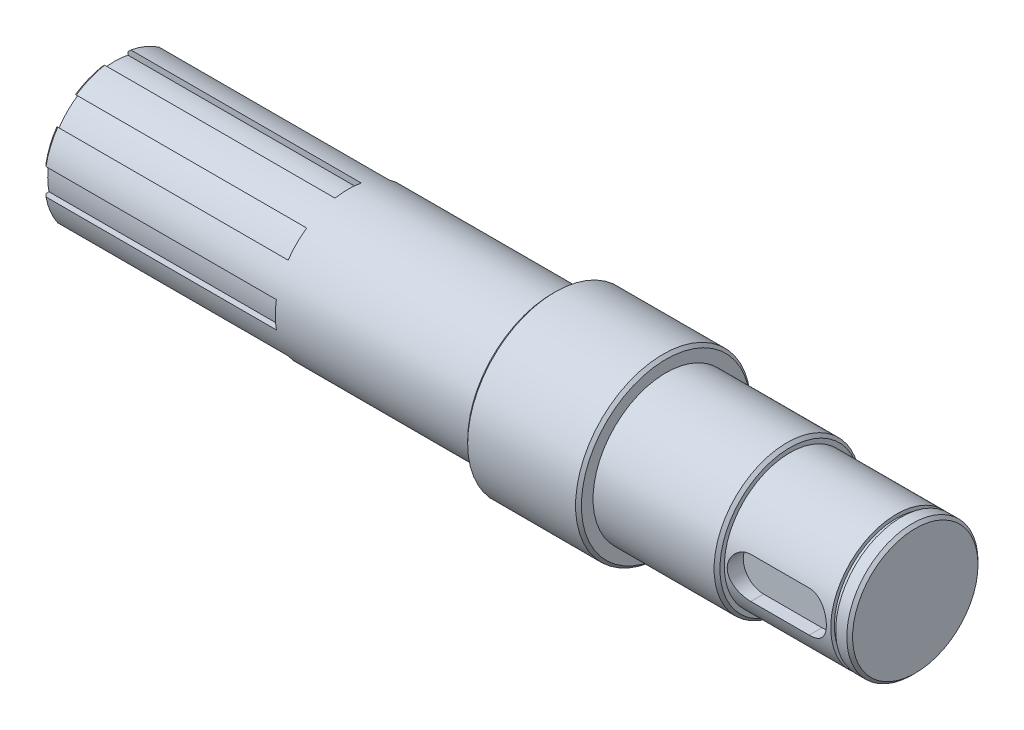
from build123d import *

# Parameters (mm, degrees)
CHAMFER_1_SIZE      = 1
CUT_EXTRUDE_START   = 1.7
SKETCH_2_R          = 22.5
SKETCH_2_R_2        = 21.25
CUT_EXTRUDE_1_DEPTH = 1.7
CUT_EXTRUDE_2_DEPTH = 5.5
CUT_EXTRUDE_START_2 = -80
CUT_EXTRUDE_3_DEPTH = 80
CHAMFER_2_SIZE      = 1


with BuildPart() as part:
    # 草图1 → 旋转1 (revolve)
    with BuildSketch(Plane.XY, mode=Mode.PRIVATE) as revolve_1_sk:
        Polygon((0, 0), (0, 25), (150, 25), (150, 30), (189, 30), (189, 25), (231.5, 25), (231.5, 22.5), (274.5, 22.5), (274.5, 0), align=None)
    revolve(revolve_1_sk.sketch.rotate(Axis((274.5, 0, 0), (-1, 0, 0)), 90), axis=Axis((274.5, 0, 0), (-1, 0, 0)))

    # 倒角1
    chamfer_1_edges = [part.edges().sort_by_distance(p)[0] for p in [
        (274.5, 0, 22.5),
        (231.5, 0, 25),
        (189, 0, 30),
        (150, 0, 30),
    ]]
    chamfer(chamfer_1_edges, length=CHAMFER_1_SIZE)

    # 草图2 → 切除-拉伸1 (cut)
    with BuildSketch(Plane(origin=(268, 0, 0), x_dir=(0, 0, -1), z_dir=(1, 0, 0)).offset(CUT_EXTRUDE_START)):
        Circle(SKETCH_2_R)
        Circle(SKETCH_2_R_2, mode=Mode.SUBTRACT)
    extrude(amount=-CUT_EXTRUDE_1_DEPTH, mode=Mode.SUBTRACT)

    # 草图3 → 切除-拉伸2 (cut)
    with BuildSketch(Plane.XY.offset(22.5)):
        with BuildLine():
            Line((239.5, 7), (259.5, 7))
            ThreePointArc((259.5, 7), (266.5, 0), (259.5, -7))
            Line((259.5, -7), (239.5, -7))
            ThreePointArc((239.5, -7), (232.5, 0), (239.5, 7))
        make_face()
    extrude(amount=-CUT_EXTRUDE_2_DEPTH, mode=Mode.SUBTRACT)

    # 草图4 → 切除-拉伸3 (cut)
    with BuildSketch(Plane.ZY.offset(CUT_EXTRUDE_START_2)):
        with BuildLine():
            Line((-4.5, 24.591665255), (-4.5, 22.555487137))
            ThreePointArc((-4.5, 22.555487137), (0, 23), (4.5, 22.555487137))
            Line((4.5, 22.555487137), (4.5, 24.591665255))
            ThreePointArc((4.5, 24.591665255), (0, 25), (-4.5, 24.591665255))
        make_face()
        with BuildLine():
            Line((20.570913778, 14.206952747), (19.131118423, 12.767157392))
            ThreePointArc((19.131118423, 12.767157392), (16.263455967, 16.263455967), (12.767157392, 19.131118423))
            Line((12.767157392, 19.131118423), (14.206952747, 20.570913778))
            ThreePointArc((14.206952747, 20.570913778), (17.67766953, 17.67766953), (20.570913778, 14.206952747))
        make_face()
        with BuildLine():
            Line((24.591665255, -4.5), (22.555487137, -4.5))
            ThreePointArc((22.555487137, -4.5), (23, 0), (22.555487137, 4.5))
            Line((22.555487137, 4.5), (24.591665255, 4.5))
            ThreePointArc((24.591665255, 4.5), (25, 0), (24.591665255, -4.5))
        make_face()
        with BuildLine():
            Line((14.206952747, -20.570913778), (12.767157392, -19.131118423))
            ThreePointArc((12.767157392, -19.131118423), (16.263455967, -16.263455967), (19.131118423, -12.767157392))
            Line((19.131118423, -12.767157392), (20.570913778, -14.206952747))
            ThreePointArc((20.570913778, -14.206952747), (17.67766953, -17.67766953), (14.206952747, -20.570913778))
        make_face()
        with BuildLine():
            Line((-4.5, -24.591665255), (-4.5, -22.555487137))
            ThreePointArc((-4.5, -22.555487137), (0, -23), (4.5, -22.555487137))
            Line((4.5, -22.555487137), (4.5, -24.591665255))
            ThreePointArc((4.5, -24.591665255), (0, -25), (-4.5, -24.591665255))
        make_face()
        with BuildLine():
            Line((-20.570913778, -14.206952747), (-19.131118423, -12.767157392))
            ThreePointArc((-19.131118423, -12.767157392), (-16.263455967, -16.263455967), (-12.767157392, -19.131118423))
            Line((-12.767157392, -19.131118423), (-14.206952747, -20.570913778))
            ThreePointArc((-14.206952747, -20.570913778), (-17.67766953, -17.67766953), (-20.570913778, -14.206952747))
        make_face()
        with BuildLine():
            Line((-24.591665255, 4.5), (-22.555487137, 4.5))
            ThreePointArc((-22.555487137, 4.5), (-23, 0), (-22.555487137, -4.5))
            Line((-22.555487137, -4.5), (-24.591665255, -4.5))
            ThreePointArc((-24.591665255, -4.5), (-25, 0), (-24.591665255, 4.5))
        make_face()
        with BuildLine():
            Line((-14.206952747, 20.570913778), (-12.767157392, 19.131118423))
            ThreePointArc((-12.767157392, 19.131118423), (-16.263455967, 16.263455967), (-19.131118423, 12.767157392))
            Line((-19.131118423, 12.767157392), (-20.570913778, 14.206952747))
            ThreePointArc((-20.570913778, 14.206952747), (-17.67766953, 17.67766953), (-14.206952747, 20.570913778))
        make_face()
    extrude(amount=CUT_EXTRUDE_3_DEPTH, mode=Mode.SUBTRACT)

    # 倒角2
    chamfer_2_edges = [part.edges().sort_by_distance(p)[0] for p in [
        (0, 23.096988313, 9.567085809),
        (0, 9.567085809, 23.096988313),
        (0, -9.567085809, 23.096988313),
        (0, -23.096988313, 9.567085809),
        (0, -23.096988313, -9.567085809),
        (0, -9.567085809, -23.096988313),
        (0, 9.567085809, -23.096988313),
        (0, 23.096988313, -9.567085809),
    ]]
    chamfer(chamfer_2_edges, length=CHAMFER_2_SIZE)


solid = part.part
